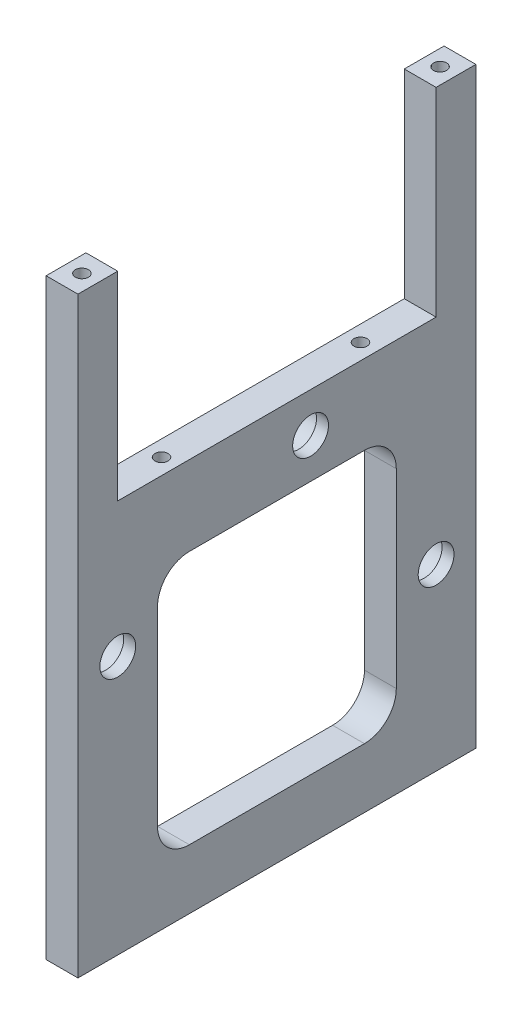
from build123d import *

# Parameters (mm, degrees)
SKETCH1_W               = 100
SKETCH1_H               = 98.830024952
SKETCH1_R               = 4.5
SKETCH1_W_2             = 60
SKETCH1_H_2             = 63.830024952
BOSS_EXTRUDE1_DEPTH     = 8
SKETCH4_R               = 5.55
CUT_EXTRUDE2_DEPTH      = 5
FILLET2_R               = 8
M2_5_TAPPED_HOLE1_D     = 2.05
M2_5_TAPPED_HOLE1_DEPTH = 6
M2_5_TAPPED_HOLE1_TIP   = 0.615882135
SKETCH11_R              = 1
CUT_EXTRUDE3_DEPTH      = 10
M4_TAPPED_HOLE1_D       = 3.3
M4_TAPPED_HOLE1_DEPTH   = 11.5
M4_TAPPED_HOLE1_TIP     = 0.991420021
SKETCH21_W              = 8
SKETCH21_H              = 10
BOSS_EXTRUDE2_DEPTH     = 50
M4_TAPPED_HOLE5_D       = 3.3
M4_TAPPED_HOLE5_DEPTH   = 8
M4_TAPPED_HOLE5_TIP     = 0.991420021
M4_TAPPED_HOLE6_D       = 3.3
M4_TAPPED_HOLE6_DEPTH   = 8
M4_TAPPED_HOLE6_TIP     = 0.991420021


with BuildPart() as part:
    # Sketch1 → Boss-Extrude1 (new body)
    with BuildSketch(Plane(origin=(0, 0, 0), x_dir=(0, 0, -1), z_dir=(1, 0, 0))):
        with Locations((9.943041263, -14.350886945)):
            Rectangle(SKETCH1_W, SKETCH1_H)
        with Locations((-30.056958737, 1.234100579)):
            Circle(SKETCH1_R, mode=Mode.SUBTRACT)
        with Locations((18.400547501, 25.064125531)):
            Circle(SKETCH1_R, mode=Mode.SUBTRACT)
        with Locations((49.943041263, -18.765899421)):
            Circle(SKETCH1_R, mode=Mode.SUBTRACT)
        with Locations((9.943041263, -16.850886945)):
            Rectangle(SKETCH1_W_2, SKETCH1_H_2, mode=Mode.SUBTRACT)
    extrude(amount=BOSS_EXTRUDE1_DEPTH)

    # Sketch4 → Cut-Extrude2 (cut)
    with BuildSketch(Plane.ZY):
        with Locations((-18.400547501, 25.064125531)):
            Circle(SKETCH4_R)
        with Locations((30.056958737, 1.234100579)):
            Circle(SKETCH4_R)
        with Locations((-49.943041263, -18.765899421)):
            Circle(SKETCH4_R)
    extrude(amount=-CUT_EXTRUDE2_DEPTH, mode=Mode.SUBTRACT)

    # Fillet2
    fillet2_edges = [part.edges().sort_by_distance(p)[0] for p in [
        (4, 15.064125531, 20.056958737),
        (4, -48.765899421, 20.056958737),
        (4, -48.765899421, -39.943041263),
        (4, 15.064125531, -39.943041263),
    ]]
    fillet(fillet2_edges, radius=FILLET2_R)

    # M2.5 Tapped Hole1
    with Locations(Plane(origin=(0, 25.064125531, -26.150547501), x_dir=(0, 0, -1), z_dir=(-1, 0, 0))):
        with Locations((0, 0), (-15.5, 0), (23.792493762, 36.080024952), (23.792493762, 51.580024952), (-56.207506238, 16.080024952), (-56.207506238, 31.580024952)):
            Hole(M2_5_TAPPED_HOLE1_D / 2, depth=M2_5_TAPPED_HOLE1_DEPTH)
            with Locations((0, 0, -(M2_5_TAPPED_HOLE1_DEPTH + M2_5_TAPPED_HOLE1_TIP / 2))):  # 118° drill point
                Cone(0, M2_5_TAPPED_HOLE1_D / 2, M2_5_TAPPED_HOLE1_TIP, mode=Mode.SUBTRACT)

    # Sketch11 → Cut-Extrude3 (cut)
    with BuildSketch(Plane.XZ.offset(63.765899421)):
        with Locations(Location((4.001919783, -44.943041263, 0), (0, 0, 270))):
            Circle(SKETCH11_R)
        with Locations(Location((4.001919783, 30.056958737, 0), (0, 0, 270))):
            Circle(SKETCH11_R)
        with Locations(Location((4.001919783, -19.943041263, 0), (0, 0, 270))):
            Circle(SKETCH11_R)
        with Locations(Location((4.001919783, 5.056958737, 0), (0, 0, 270))):
            Circle(SKETCH11_R)
    extrude(amount=-CUT_EXTRUDE3_DEPTH, mode=Mode.SUBTRACT)

    # M4 Tapped Hole1
    with Locations(Plane(origin=(0, -63.765899421, 0), x_dir=(-1, 0, 0), z_dir=(0, -1, 0))):
        with Locations((-4.001919783, 44.943041263), (-4.001919783, 19.943041263), (-4.001919783, -5.056958737), (-4.001919783, -30.056958737)):
            Hole(M4_TAPPED_HOLE1_D / 2, depth=M4_TAPPED_HOLE1_DEPTH)
            with Locations((0, 0, -(M4_TAPPED_HOLE1_DEPTH + M4_TAPPED_HOLE1_TIP / 2))):  # 118° drill point
                Cone(0, M4_TAPPED_HOLE1_D / 2, M4_TAPPED_HOLE1_TIP, mode=Mode.SUBTRACT)

    # Sketch21 → Boss-Extrude2 (add)
    with BuildSketch(Plane(origin=(0, 35.064125531, 0), x_dir=(1, 0, 0), z_dir=(0, 1, 0))):
        with Locations((4, 54.943041263)):
            Rectangle(SKETCH21_W, SKETCH21_H)
        with Locations((4, -35.056958737)):
            Rectangle(SKETCH21_W, SKETCH21_H)
    extrude(amount=BOSS_EXTRUDE2_DEPTH)

    # M4 Tapped Hole5
    with Locations(Plane(origin=(0, 85.064125531, 0), x_dir=(1, 0, 0), z_dir=(0, 1, 0))):
        with Locations((4, 54.943041263), (4, -35.056958737)):
            Hole(M4_TAPPED_HOLE5_D / 2, depth=M4_TAPPED_HOLE5_DEPTH)
            with Locations((0, 0, -(M4_TAPPED_HOLE5_DEPTH + M4_TAPPED_HOLE5_TIP / 2))):  # 118° drill point
                Cone(0, M4_TAPPED_HOLE5_D / 2, M4_TAPPED_HOLE5_TIP, mode=Mode.SUBTRACT)

    # M4 Tapped Hole6
    with Locations(Plane(origin=(0, 35.064125531, 0), x_dir=(1, 0, 0), z_dir=(0, 1, 0))):
        with Locations((4, 34.943041263), (4, -15.056958737)):
            Hole(M4_TAPPED_HOLE6_D / 2, depth=M4_TAPPED_HOLE6_DEPTH)
            with Locations((0, 0, -(M4_TAPPED_HOLE6_DEPTH + M4_TAPPED_HOLE6_TIP / 2))):  # 118° drill point
                Cone(0, M4_TAPPED_HOLE6_D / 2, M4_TAPPED_HOLE6_TIP, mode=Mode.SUBTRACT)


solid = part.part
